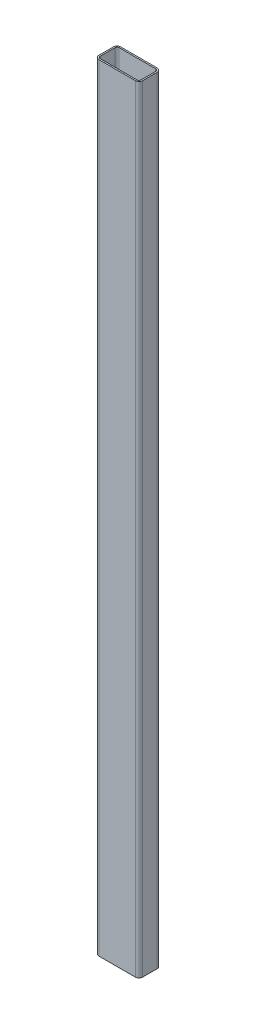
SolidWorks part; units mm, degrees
ref_plane "Front Plane" through (0, 0, 0) normal (0, 0, 1) x (1, 0, 0)
ref_plane "Top Plane" through (0, 0, 0) normal (0, 1, 0) x (1, 0, 0)
ref_plane "Right Plane" through (0, 0, 0) normal (1, 0, 0) x (0, 0, -1)
other "Configuration Table"
sketch "Sketch1" plane through (0, 0, 0) normal (0, 1, 0) x (1, 0, 0)
  line L1 (-50, 30) -> (50, 30)
  line L2 (-60, 20) -> (-60, -20)
  line L3 (-50, -30) -> (50, -30)
  line L4 (60, 20) -> (60, -20)
  line L5 (-60, 30) -> (60, -30) construction
  line L6 (-60, -30) -> (60, 30) construction
  arc A0 (50, 30) -> (60, 20) centre (50, 20) cw
  arc A1 (50, -30) -> (60, -20) centre (50, -20) ccw
  arc A2 (-60, -20) -> (-50, -30) centre (-50, -20) ccw
  arc A3 (-50, 30) -> (-60, 20) centre (-50, 20) ccw
  point P0 (0, 0)
  dimension "D3" = 10
  dimension "D1" = 120
  dimension "D2" = 60
extrude "Extrude-Thin1" add sketch "Sketch1" along normal mid plane 2124 thin
